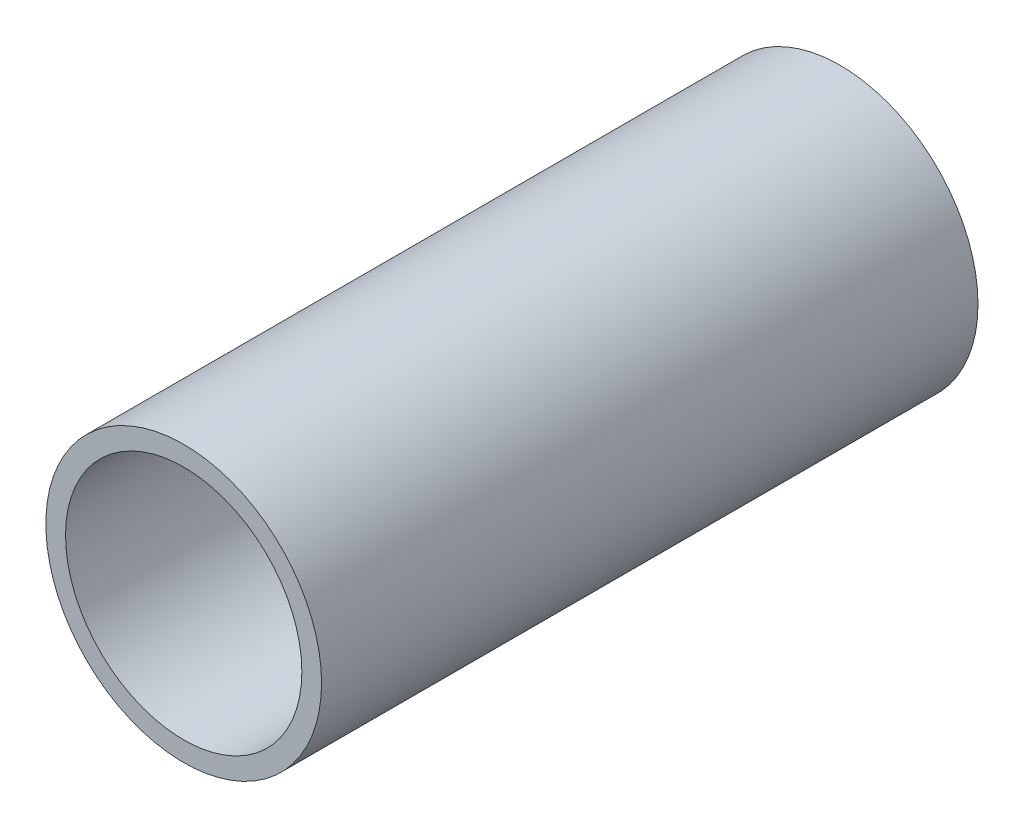
SolidWorks part; units mm, degrees
ref_plane "Front Plane" through (0, 0, 0) normal (0, 0, 1) x (1, 0, 0)
ref_plane "Top Plane" through (0, 0, 0) normal (0, 1, 0) x (1, 0, 0)
ref_plane "Right Plane" through (0, 0, 0) normal (1, 0, 0) x (0, 0, -1)
sketch "Sketch 1" plane through (0, 0, 0) normal (0, 0, 1) x (1, 0, 0)
  circle A0 centre (0, 0) radius 21
  circle A1 centre (0, 0) radius 18
  dimension "D1" = 42
  dimension "D2" = 3
extrude "Boss-Extrude 1" add sketch "Sketch 1" along normal blind 100
